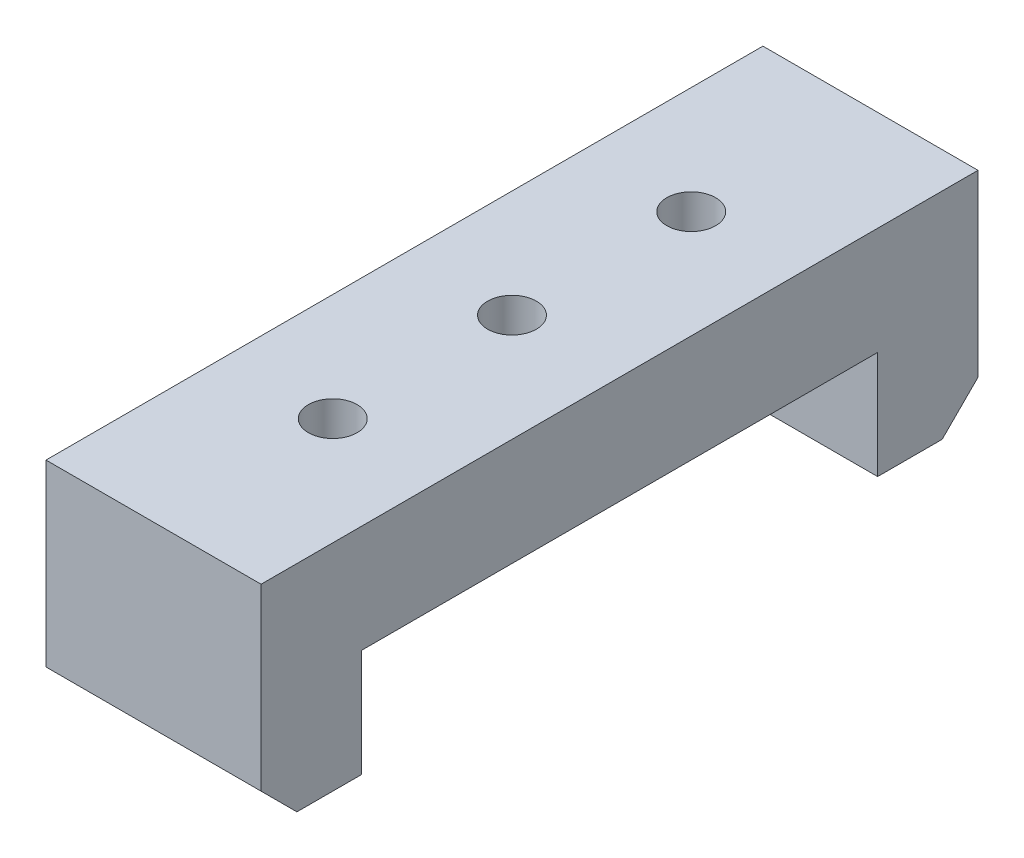
from build123d import *

# Parameters (mm, degrees)
SKETCH_1_W             = 100
SKETCH_1_H             = 30
EXTRUDE_1_DEPTH        = 30
SKETCH_2_W             = 72
SKETCH_2_H             = 15
CUT_EXTRUDE_1_DEPTH    = 15.5
HOLE_WIZARD_M8_1_D     = 6.8
HOLE_WIZARD_M8_1_DEPTH = 10
HOLE_WIZARD_M8_1_TIP   = 2.042926105
HOLE_WIZARD_M5_1_D     = 4.2
CHAMFER_1_SIZE         = 5


with BuildPart() as part:
    # 草图1 → 凸台-拉伸1 (new body)
    with BuildSketch(Plane(origin=(0, 0, 0), x_dir=(0, 0, -1), z_dir=(1, 0, 0))):
        Rectangle(SKETCH_1_W, SKETCH_1_H)
    extrude(amount=EXTRUDE_1_DEPTH)

    # 草图2 → 切除-拉伸1 (cut)
    with BuildSketch(Plane(origin=(30, 0, 0), x_dir=(0, 0, -1), z_dir=(1, 0, 0))):
        with Locations((0, -7.5)):
            Rectangle(SKETCH_2_W, SKETCH_2_H)
    extrude(amount=-CUT_EXTRUDE_1_DEPTH, mode=Mode.SUBTRACT)

    # M8 螺纹孔1
    with Locations(Plane(origin=(0, 15, 0), x_dir=(1, 0, 0), z_dir=(0, 1, 0))):
        with Locations((15, 0), (15, 25), (15, -25)):
            Hole(HOLE_WIZARD_M8_1_D / 2, depth=HOLE_WIZARD_M8_1_DEPTH)
            with Locations((0, 0, -(HOLE_WIZARD_M8_1_DEPTH + HOLE_WIZARD_M8_1_TIP / 2))):  # 118° drill point
                Cone(0, HOLE_WIZARD_M8_1_D / 2, HOLE_WIZARD_M8_1_TIP, mode=Mode.SUBTRACT)

    # M5 螺纹孔1 (through all)
    with Locations(Plane(origin=(14.5, 0, 0), x_dir=(0, 0, -1), z_dir=(1, 0, 0))):
        with Locations((-20, -8), (0, -8), (20, -8)):
            Hole(HOLE_WIZARD_M5_1_D / 2)

    # 倒角1
    chamfer_1_edges = [part.edges().sort_by_distance(p)[0] for p in [
        (15, -15, -50),
        (15, -15, 50),
    ]]
    chamfer(chamfer_1_edges, length=CHAMFER_1_SIZE)


solid = part.part
